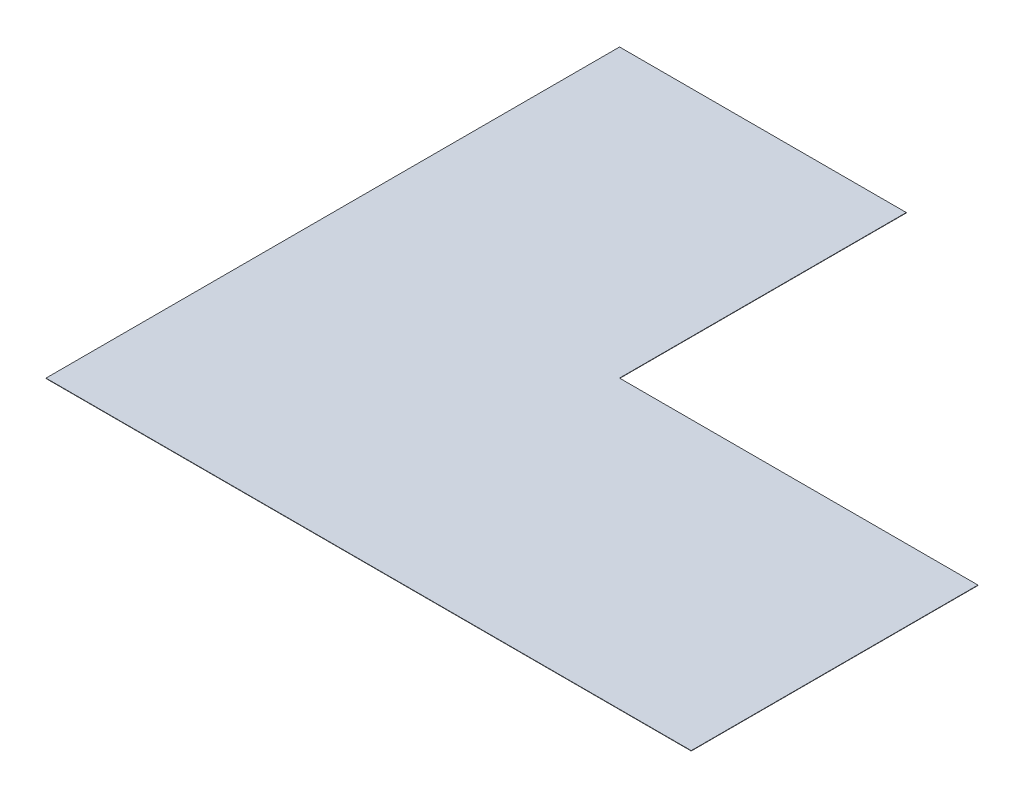
from build123d import *

# Parameters (mm, degrees)
BOSS_EXTRUDE1_DEPTH = 1


with BuildPart() as part:
    # Sketch1 → Boss-Extrude1 (new body)
    with BuildSketch(Plane(origin=(0, 0, 0), x_dir=(1, 0, 0), z_dir=(0, 1, 0))):
        Polygon((-900, -800), (900, -800), (900, 0), (0, 0), (-100, 0), (-100, 800), (-900, 800), align=None)
    extrude(amount=BOSS_EXTRUDE1_DEPTH)


solid = part.part
